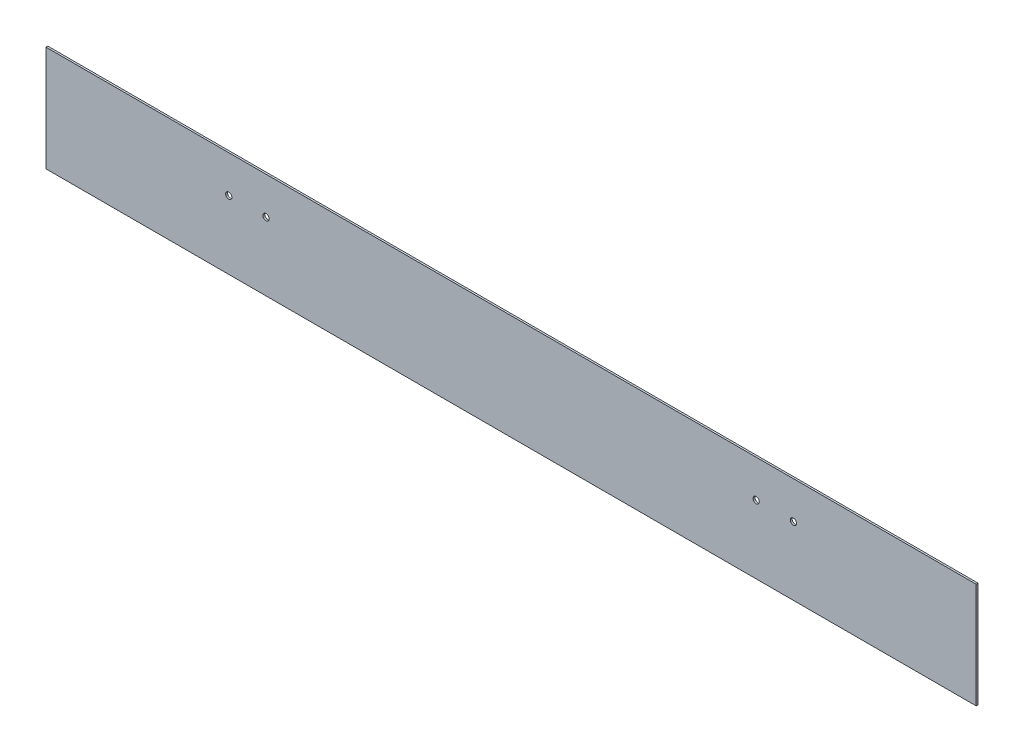
from build123d import *

# Parameters (mm, degrees)
SKETCH_1_W          = 1500
SKETCH_1_H          = 160
EXTRUDE_1_DEPTH     = 3
SKETCH_3_R          = 5
CUT_EXTRUDE_1_DEPTH = 755.260565057
SKETCH_7_W          = 1500
SKETCH_7_H          = 3
EXTRUDE_2_DEPTH     = 10


with BuildPart() as part:
    # 草图1 → 凸台-拉伸1 (new body)
    with BuildSketch(Plane.XY):
        Rectangle(SKETCH_1_W, SKETCH_1_H)
    extrude(amount=EXTRUDE_1_DEPTH)

    # 草图3 → 切除-拉伸1 (cut, symmetric)
    with BuildSketch(Plane.XY.offset(3)):
        with Locations((-455.26, 30)):
            Circle(SKETCH_3_R)
        with Locations((-395.26, 30)):
            Circle(SKETCH_3_R)
    cut_extrude_1 = extrude(amount=CUT_EXTRUDE_1_DEPTH, both=True, mode=Mode.SUBTRACT)

    # 镜向1: 切除-拉伸1 across plane
    add(cut_extrude_1.mirror(Plane(origin=(0, 0, 0), x_dir=(0, 0, 1), z_dir=(1, 0, 0))), mode=Mode.SUBTRACT)

    # 草图7 → 凸台-拉伸2 (add)
    with BuildSketch(Plane(origin=(0, 80, 0), x_dir=(1, 0, 0), z_dir=(0, 1, 0))):
        with Locations((0, -1.5)):
            Rectangle(SKETCH_7_W, SKETCH_7_H)
    extrude(amount=EXTRUDE_2_DEPTH)


solid = part.part
